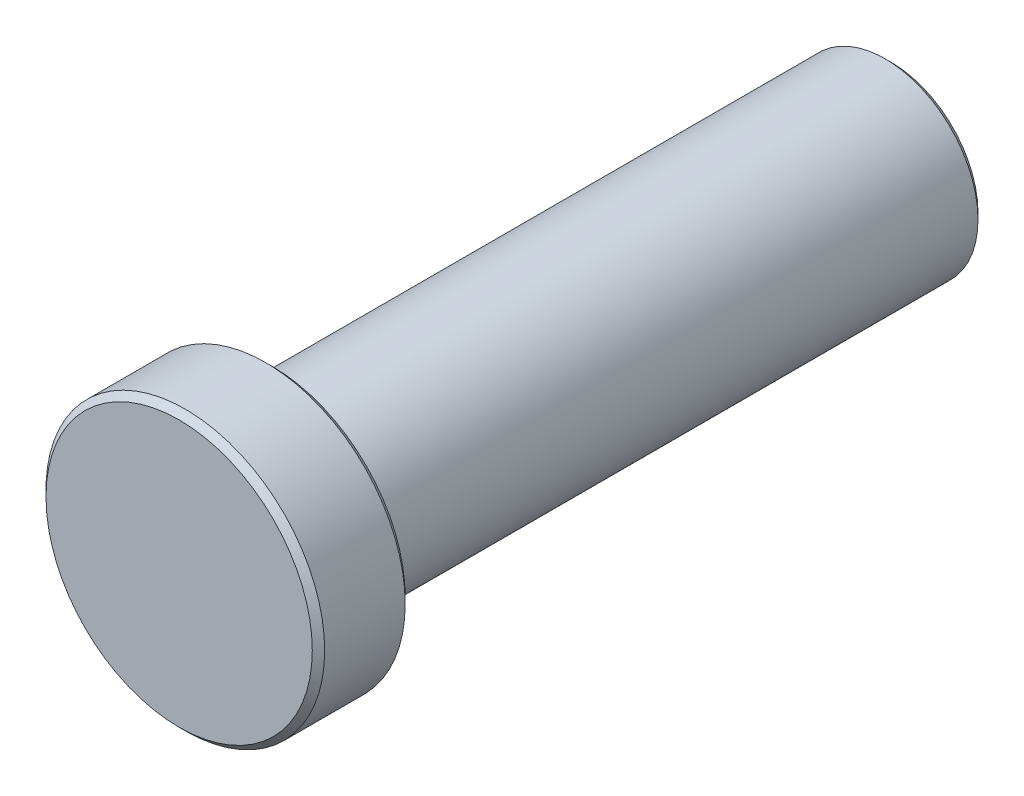
from build123d import *

# Parameters (mm, degrees)
SKETCH1_R           = 3
BOSS_EXTRUDE1_DEPTH = 20
SKETCH2_R           = 4.5
BOSS_EXTRUDE2_DEPTH = 3
CHAMFER1_SIZE       = 0.2


with BuildPart() as part:
    # Sketch1 → Boss-Extrude1 (new body)
    with BuildSketch(Plane.XY):
        Circle(SKETCH1_R)
    extrude(amount=BOSS_EXTRUDE1_DEPTH)

    # Sketch2 → Boss-Extrude2 (add)
    with BuildSketch(Plane.XY.offset(20)):
        Circle(SKETCH2_R)
    extrude(amount=BOSS_EXTRUDE2_DEPTH)

    # Chamfer1
    chamfer1_edges = [part.edges().sort_by_distance(p)[0] for p in [
        (-3, 0, 0),
        (-4.5, 0, 20),
        (-4.5, 0, 23),
    ]]
    chamfer(chamfer1_edges, length=CHAMFER1_SIZE)


solid = part.part
